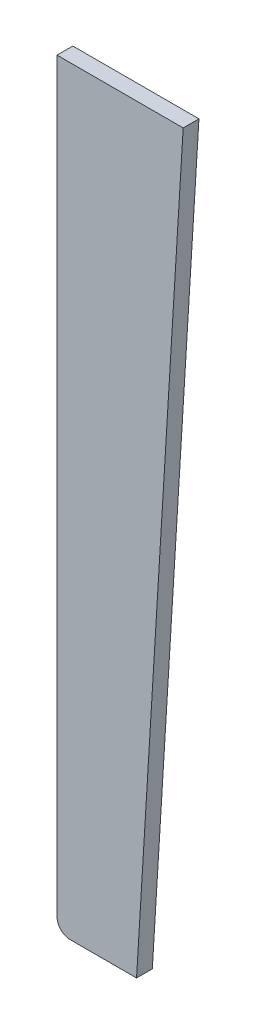
SolidWorks part; units mm, degrees
ref_plane "Front Plane" through (0, 0, 0) normal (0, 0, 1) x (1, 0, 0)
ref_plane "Top Plane" through (0, 0, 0) normal (0, 1, 0) x (1, 0, 0)
ref_plane "Right Plane" through (0, 0, 0) normal (1, 0, 0) x (0, 0, -1)
sketch "Sketch1" plane through (0, 0, 0) normal (0, 0, 1) x (1, 0, 0)
  line L0 (0, 10) -> (0, 578)
  line L1 (0, 578) -> (96, 578)
  line L2 (96, 578) -> (60.5, 0)
  line L3 (60.5, 0) -> (10, 0)
  arc A0 (0, 10) -> (10, 0) centre (10, 10) ccw
  point P7 (0, 0)
  dimension "D4" = 10
  dimension "D1" = 96
  dimension "D2" = 578
  dimension "D3" = 60.5
extrude "Boss-Extrude1" add sketch "Sketch1" along normal blind 12
